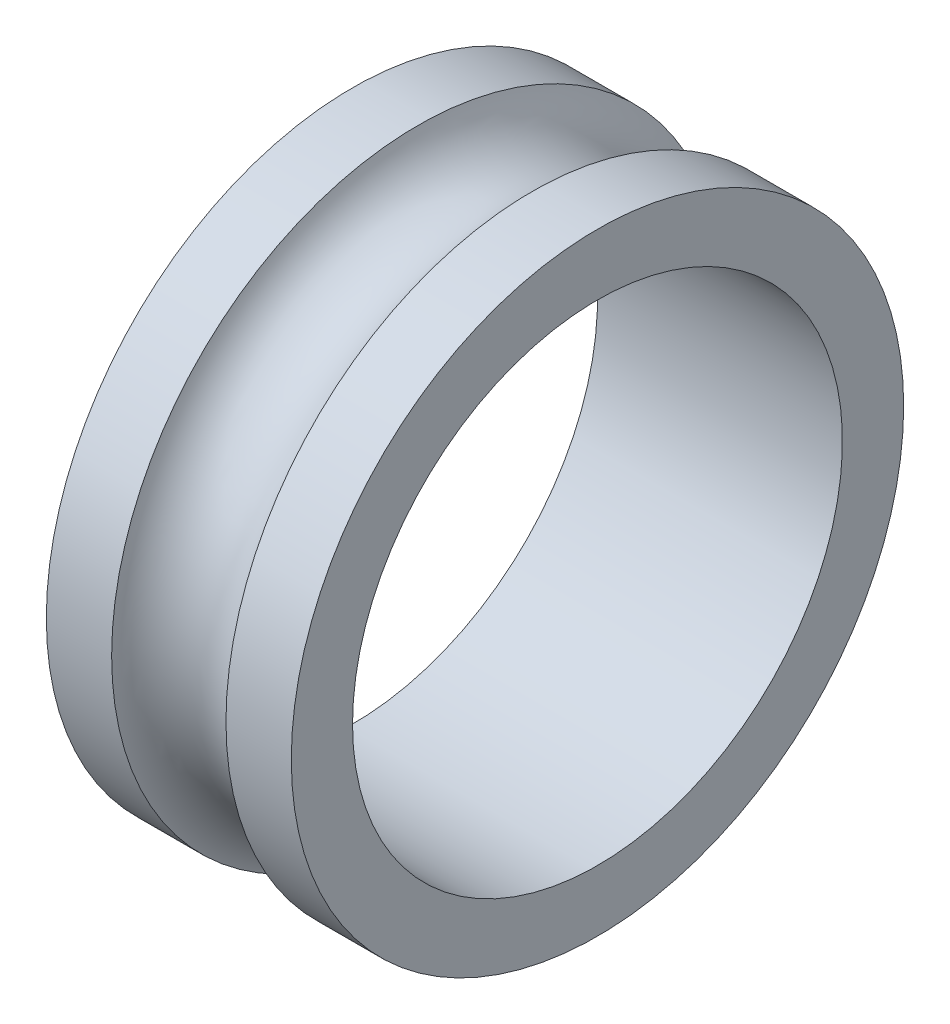
from build123d import *


with BuildPart() as part:
    # Sketch1 → Revolve1 (revolve)
    with BuildSketch(Plane.XY, mode=Mode.PRIVATE) as revolve1_sk:
        with BuildLine():
            Line((0, 6), (0, 7.5))
            Line((0, 7.5), (1.6, 7.5))
            ThreePointArc((1.6, 7.5), (3, 6.5), (4.4, 7.5))
            Line((4.4, 7.5), (6, 7.5))
            Line((6, 7.5), (6, 6))
            Line((6, 6), (0, 6))
        make_face()
    revolve(revolve1_sk.sketch.rotate(Axis((0, 0, 0), (1, 0, 0)), 90), axis=Axis((0, 0, 0), (1, 0, 0)))


solid = part.part
